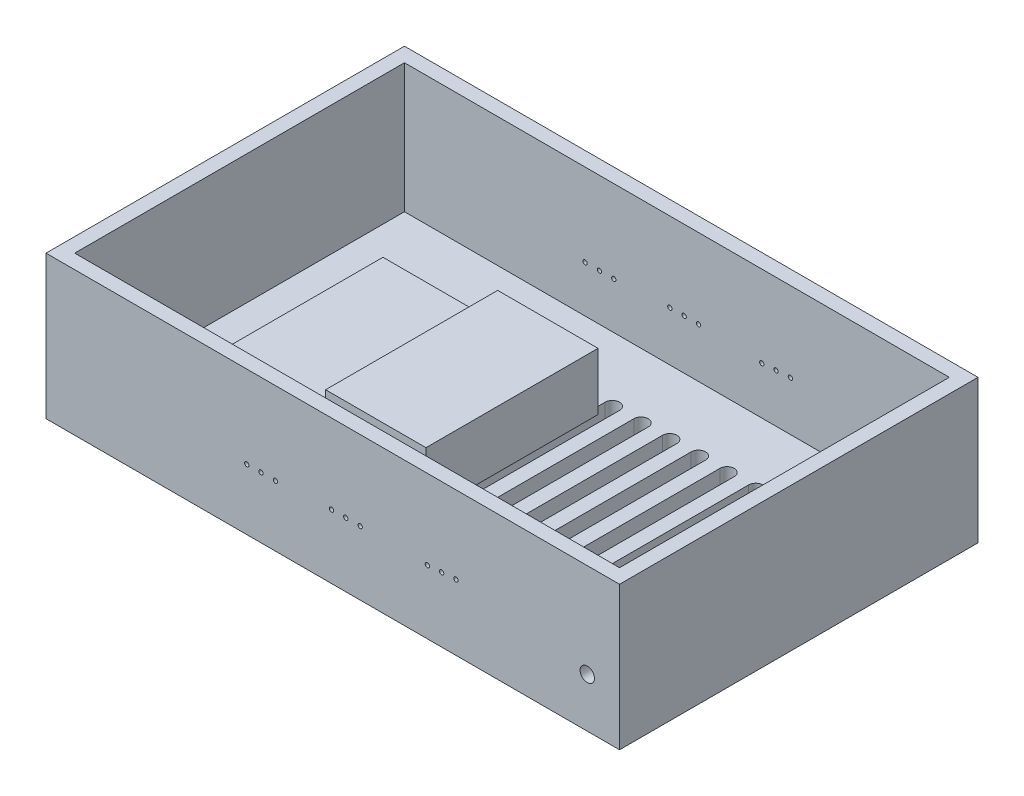
from build123d import *

# Parameters (mm, degrees)
SKETCH1_W           = 400
SKETCH1_H           = 100
BOSS_EXTRUDE1_DEPTH = 125
SHELL1_T            = -10
SKETCH2_R           = 1.5
CUT_EXTRUDE1_DEPTH  = 20
SKETCH6_W           = 150
SKETCH6_H           = 120
BOSS_EXTRUDE2_DEPTH = 20
CUT_EXTRUDE4_DEPTH  = 40
SKETCH10_W          = 70
SKETCH10_H          = 120
BOSS_EXTRUDE4_DEPTH = 20
SKETCH11_R          = 5
CUT_EXTRUDE5_DEPTH  = 20
SKETCH12_R          = 5
CUT_EXTRUDE6_DEPTH  = 20
SKETCH13_R          = 1.5
CUT_EXTRUDE7_DEPTH  = 20


with BuildPart() as part:
    # Sketch1 → Boss-Extrude1 (new, symmetric)
    with BuildSketch(Plane.XY):
        Rectangle(SKETCH1_W, SKETCH1_H)
    extrude(amount=BOSS_EXTRUDE1_DEPTH, both=True)

    # Shell1
    shell1_openings = [part.faces().sort_by_distance(p)[0] for p in [
        (0, 50, 0),
    ]]
    offset(amount=SHELL1_T, openings=shell1_openings, kind=Kind.INTERSECTION)

    # Sketch2 → Cut-Extrude1 (cut)
    with BuildSketch(Plane.XY.offset(125)):
        with Locations((-60, -7.5)):
            Circle(SKETCH2_R)
        with Locations((-50.069563203, -7.468939407)):
            Circle(SKETCH2_R)
        with Locations((-40, -7.499999981)):
            Circle(SKETCH2_R)
        with Locations((-0.893423466, -5.30577502)):
            Circle(SKETCH2_R)
        with Locations((9.032429625, -5.272668135)):
            Circle(SKETCH2_R)
        with Locations((19.106576534, -5.305775001)):
            Circle(SKETCH2_R)
        with Locations((65.964532087, -5.478731969)):
            Circle(SKETCH2_R)
        with Locations((75.941621303, -4.802203506)):
            Circle(SKETCH2_R)
        with Locations((85.91871052, -4.125675044)):
            Circle(SKETCH2_R)
    extrude(amount=-CUT_EXTRUDE1_DEPTH, mode=Mode.SUBTRACT)

    # Sketch6 → Boss-Extrude2 (add)
    with BuildSketch(Plane(origin=(0, -40, 0), x_dir=(1, 0, 0), z_dir=(0, 1, 0))):
        with Locations((-75, 0)):
            Rectangle(SKETCH6_W, SKETCH6_H)
    extrude(amount=BOSS_EXTRUDE2_DEPTH)

    # Sketch9 → Cut-Extrude4 (cut)
    with BuildSketch(Plane(origin=(0, -40, 0), x_dir=(1, 0, 0), z_dir=(0, 1, 0))):
        with BuildLine():
            Line((105, 70), (105, -70))
            ThreePointArc((105, -70), (100, -75), (95, -70))
            Line((95, -70), (95, 70))
            ThreePointArc((95, 70), (100, 75), (105, 70))
        make_face()
        with BuildLine():
            Line((85, 70), (85, -70))
            ThreePointArc((85, -70), (80, -75), (75, -70))
            Line((75, -70), (75, 70))
            ThreePointArc((75, 70), (80, 75), (85, 70))
        make_face()
        with BuildLine():
            Line((65, 70), (65, -70))
            ThreePointArc((65, -70), (60, -75), (55, -70))
            Line((55, -70), (55, 70))
            ThreePointArc((55, 70), (60, 75), (65, 70))
        make_face()
        with BuildLine():
            Line((45, 70), (45, -70))
            ThreePointArc((45, -70), (40, -75), (35, -70))
            Line((35, -70), (35, 70))
            ThreePointArc((35, 70), (40, 75), (45, 70))
        make_face()
        with BuildLine():
            Line((25, 70), (25, -70))
            ThreePointArc((25, -70), (20, -75), (15, -70))
            Line((15, -70), (15, 70))
            ThreePointArc((15, 70), (20, 75), (25, 70))
        make_face()
        with BuildLine():
            Line((5, 70), (5, -70))
            ThreePointArc((5, -70), (0, -75), (-5, -70))
            Line((-5, -70), (-5, 70))
            ThreePointArc((-5, 70), (0, 75), (5, 70))
        make_face()
        with BuildLine():
            Line((-15, 70), (-15, -70))
            ThreePointArc((-15, -70), (-20, -75), (-25, -70))
            Line((-25, -70), (-25, 70))
            ThreePointArc((-25, 70), (-20, 75), (-15, 70))
        make_face()
        with BuildLine():
            Line((-35, 70), (-35, -70))
            ThreePointArc((-35, -70), (-40, -75), (-45, -70))
            Line((-45, -70), (-45, 70))
            ThreePointArc((-45, 70), (-40, 75), (-35, 70))
        make_face()
        with BuildLine():
            Line((-55, 70), (-55, -70))
            ThreePointArc((-55, -70), (-60, -75), (-65, -70))
            Line((-65, -70), (-65, 70))
            ThreePointArc((-65, 70), (-60, 75), (-55, 70))
        make_face()
        with BuildLine():
            Line((-75, 70), (-75, -70))
            ThreePointArc((-75, -70), (-80, -75), (-85, -70))
            Line((-85, -70), (-85, 70))
            ThreePointArc((-85, 70), (-80, 75), (-75, 70))
        make_face()
        with BuildLine():
            Line((-95, 70), (-95, -70))
            ThreePointArc((-95, -70), (-100, -75), (-105, -70))
            Line((-105, -70), (-105, 70))
            ThreePointArc((-105, 70), (-100, 75), (-95, 70))
        make_face()
        with BuildLine():
            Line((-115, 70), (-115, -70))
            ThreePointArc((-115, -70), (-120, -75), (-125, -70))
            Line((-125, -70), (-125, 70))
            ThreePointArc((-125, 70), (-120, 75), (-115, 70))
        make_face()
        with BuildLine():
            Line((-135, 70), (-135, -70))
            ThreePointArc((-135, -70), (-140, -75), (-145, -70))
            Line((-145, -70), (-145, 70))
            ThreePointArc((-145, 70), (-140, 75), (-135, 70))
        make_face()
        with BuildLine():
            Line((-155, 70), (-155, -70))
            ThreePointArc((-155, -70), (-160, -75), (-165, -70))
            Line((-165, -70), (-165, 70))
            ThreePointArc((-165, 70), (-160, 75), (-155, 70))
        make_face()
    extrude(amount=-CUT_EXTRUDE4_DEPTH, mode=Mode.SUBTRACT)

    # Sketch10 → Boss-Extrude4 (add)
    with BuildSketch(Plane(origin=(0, -20, 0), x_dir=(1, 0, 0), z_dir=(0, 1, 0))):
        with Locations((-35, 0)):
            Rectangle(SKETCH10_W, SKETCH10_H)
    extrude(amount=BOSS_EXTRUDE4_DEPTH)

    # Sketch11 → Cut-Extrude5 (cut)
    with BuildSketch(Plane.XY.offset(125)):
        with Locations((177.51, -15.63)):
            Circle(SKETCH11_R)
    extrude(amount=-CUT_EXTRUDE5_DEPTH, mode=Mode.SUBTRACT)

    # Sketch12 → Cut-Extrude6 (cut)
    with BuildSketch(Plane(origin=(0, 0, -125), x_dir=(-1, 0, 0), z_dir=(0, 0, -1))):
        with Locations((-173.59, -15.71)):
            Circle(SKETCH12_R)
    extrude(amount=-CUT_EXTRUDE6_DEPTH, mode=Mode.SUBTRACT)

    # Sketch13 → Cut-Extrude7 (cut)
    with BuildSketch(Plane(origin=(0, 0, -125), x_dir=(-1, 0, 0), z_dir=(0, 0, -1))):
        with Locations((-79.16, -5.57)):
            Circle(SKETCH13_R)
        with Locations((-59.205821103, -6.923050088)):
            Circle(SKETCH13_R)
        with Locations((-69.182910551, -6.246525044)):
            Circle(SKETCH13_R)
        with Locations((64.01999621, -7.568935655)):
            Circle(SKETCH13_R)
        with Locations((54.01999621, -7.568935655)):
            Circle(SKETCH13_R)
        with Locations((44.01999621, -7.568935655)):
            Circle(SKETCH13_R)
        with Locations((4.913420159, -5.374710514)):
            Circle(SKETCH13_R)
        with Locations((-5.086579841, -5.374710514)):
            Circle(SKETCH13_R)
        with Locations((-15.086579841, -5.374710514)):
            Circle(SKETCH13_R)
    extrude(amount=-CUT_EXTRUDE7_DEPTH, mode=Mode.SUBTRACT)


solid = part.part
